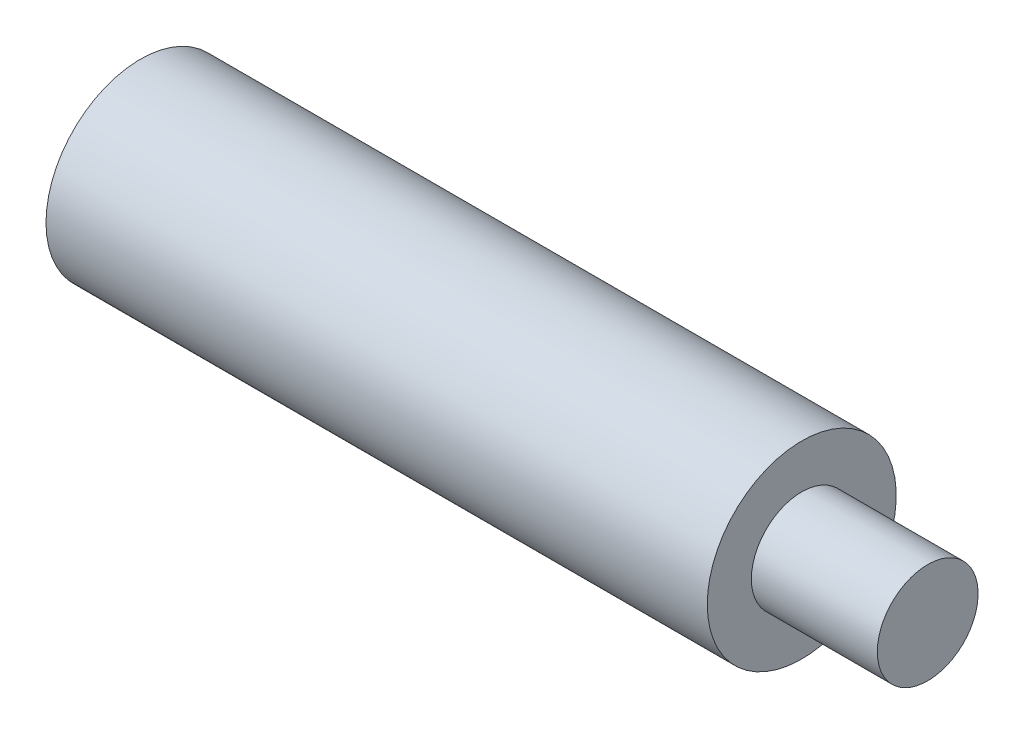
SolidWorks part; units mm, degrees
material "Q235A"
ref_plane "Front Plane" through (0, 0, 0) normal (0, 0, 1) x (1, 0, 0)
ref_plane "Top Plane" through (0, 0, 0) normal (0, 1, 0) x (1, 0, 0)
ref_plane "Right Plane" through (0, 0, 0) normal (1, 0, 0) x (0, 0, -1)
sketch "Sketch1" plane through (0, 0, 0) normal (0, 0, 1) x (1, 0, 0)
  line L0 (0, 0) -> (206.8, 0) construction
  line L1 (0, 0) -> (0, 15)
  line L2 (0, 15) -> (105, 15)
  line L3 (105, 15) -> (105, 8)
  line L4 (105, 8) -> (125, 8)
  line L5 (125, 8) -> (125, 0)
  line L6 (0, 0) -> (125, 0)
  dimension "D1" = 16
  dimension "D2" = 30
  dimension "D3" = 20
  dimension "D4" = 105
revolve "Revolve1" add sketch "Sketch1" angle 360 about L0
